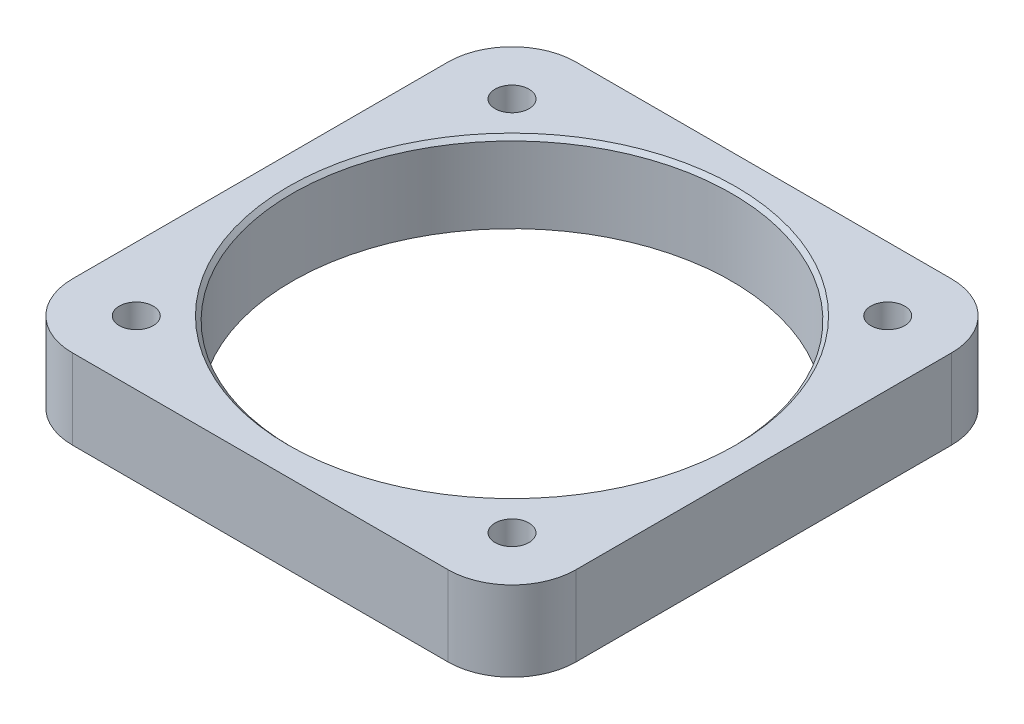
SolidWorks part; units mm, degrees
material "Q235B"
ref_plane "Front Plane" through (0, 0, 0) normal (0, 0, 1) x (1, 0, 0)
ref_plane "Top Plane" through (0, 0, 0) normal (0, 1, 0) x (1, 0, 0)
ref_plane "Right Plane" through (0, 0, 0) normal (1, 0, 0) x (0, 0, -1)
sketch "Sketch1" plane through (0, 0, 0) normal (0, 1, 0) x (1, 0, 0)
  line L1 (-47, 63) -> (47, 63)
  line L2 (-63, 47) -> (-63, -47)
  line L3 (-47, -63) -> (47, -63)
  line L4 (63, 47) -> (63, -47)
  line L5 (-63, 63) -> (63, -63) construction
  line L6 (-63, -63) -> (63, 63) construction
  circle A0 centre (0, 0) radius 55
  arc A1 (-63, -47) -> (-47, -63) centre (-47, -47) ccw
  arc A2 (47, -63) -> (63, -47) centre (47, -47) ccw
  arc A3 (47, 63) -> (63, 47) centre (47, 47) cw
  arc A4 (-47, 63) -> (-63, 47) centre (-47, 47) ccw
  point P0 (0, 0)
  dimension "D3" = 110
  dimension "D4" = 16
  dimension "D1" = 126
  dimension "D2" = 126
extrude "Boss-Extrude1" add sketch "Sketch1" along normal blind 20
sketch "Sketch2" plane through (0, 20, 0) normal (0, 1, 0) x (1, 0, 0)
  line L1 (-47, 47) -> (47, 47) construction
  line L2 (-47, 47) -> (-47, -47) construction
  line L3 (-47, -47) -> (47, -47) construction
  line L4 (47, 47) -> (47, -47) construction
  line L5 (-47, 47) -> (47, -47) construction
  line L6 (-47, -47) -> (47, 47) construction
  circle A0 centre (-47, 47) radius 4
  circle A1 centre (47, 47) radius 4
  circle A2 centre (47, -47) radius 4
  circle A3 centre (-47, -47) radius 4
  point P0 (0, 0)
  dimension "D3" = 8
  dimension "D1" = 94
  dimension "D2" = 94
extrude "Cut-Extrude1" cut sketch "Sketch2" against normal blind 3
hole_wizard "M10 Tapped Hole1" positions "Sketch3" profile "Sketch4" tap size "M10" standard "GB"
sketch "Sketch3" plane through (0, 20, 0) normal (0, 1, 0) x (1, 0, 0)
  point P0 (-47, 47)
  point P3 (47, 47)
  point P6 (47, -47)
  point P9 (-47, -47)
sketch "Sketch4" plane through (-47, 20, -47) normal (1, 0, 0) x (0, 0, 1)
  line L0 (0, 0) -> (0, 17.7837)
  line L1 (0, 17.7837) -> (4.25, 15.23)
  line L2 (4.25, 15.23) -> (4.25, 0)
  line L5 (4.25, 0) -> (0, 0)
  line L10 (0, 17.7837) -> (-4.25, 15.23) construction
  line L11 (0, -6.35) -> (0, 107.95) construction
  dimension "螺纹孔钻头直径" = 8.5
  dimension "螺纹孔钻头深度" = 15.23
  dimension "导头角度" = 118
cosmetic thread "Hole thread 1" parameters "D1"=13, "D2"=10
cosmetic thread "Hole thread 2" parameters "D1"=13, "D2"=10
cosmetic thread "Hole thread 3" parameters "D1"=13, "D2"=10
cosmetic thread "Hole thread 4" parameters "D1"=13, "D2"=10
chamfer "Chamfer1" distance 1 angle 45 1 edges at (0, 20, 55)
